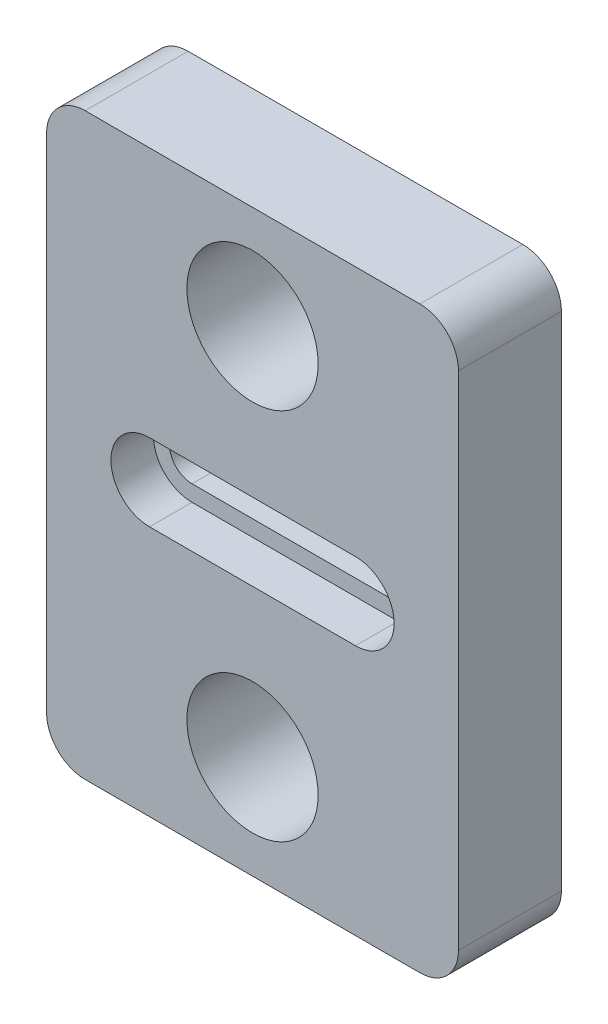
from build123d import *

# Parameters (mm, degrees)
SKETCH1_W           = 32
SKETCH1_H           = 45
BOSS_EXTRUDE1_DEPTH = 8
CUT_EXTRUDE1_DEPTH  = 29.744564704
CUT_EXTRUDE2_DEPTH  = 3.3
FILLET1_R           = 3
M12_TAPPED_HOLE2_D  = 10.2


with BuildPart() as part:
    # Sketch1 → Boss-Extrude1 (new body)
    with BuildSketch(Plane.XY):
        Rectangle(SKETCH1_W, SKETCH1_H)
    extrude(amount=BOSS_EXTRUDE1_DEPTH)

    # Sketch5 → Cut-Extrude1 (cut, through all)
    with BuildSketch(Plane.XY.offset(8)):
        with BuildLine():
            Line((-8, 1.75), (8, 1.75))
            ThreePointArc((8, 1.75), (9.75, 0), (8, -1.75))
            Line((8, -1.75), (-8, -1.75))
            ThreePointArc((-8, -1.75), (-9.75, 0), (-8, 1.75))
        make_face()
    extrude(amount=-CUT_EXTRUDE1_DEPTH, mode=Mode.SUBTRACT)

    # Sketch6 → Cut-Extrude2 (cut)
    with BuildSketch(Plane.XY.offset(8)):
        with BuildLine():
            Line((-8, 3), (8, 3))
            ThreePointArc((8, 3), (11, 0), (8, -3))
            Line((8, -3), (-8, -3))
            ThreePointArc((-8, -3), (-11, 0), (-8, 3))
        make_face()
    extrude(amount=-CUT_EXTRUDE2_DEPTH, mode=Mode.SUBTRACT)

    # Fillet1
    fillet1_edges = [part.edges().sort_by_distance(p)[0] for p in [
        (-16, 22.5, 4),
        (16, 22.5, 4),
        (16, -22.5, 4),
        (-16, -22.5, 4),
    ]]
    fillet(fillet1_edges, radius=FILLET1_R)

    # M12 Tapped Hole2 (through all)
    with Locations(Plane.XY.offset(8)):
        with Locations((0, -14.5), (0, 14.5)):
            Hole(M12_TAPPED_HOLE2_D / 2)


solid = part.part
